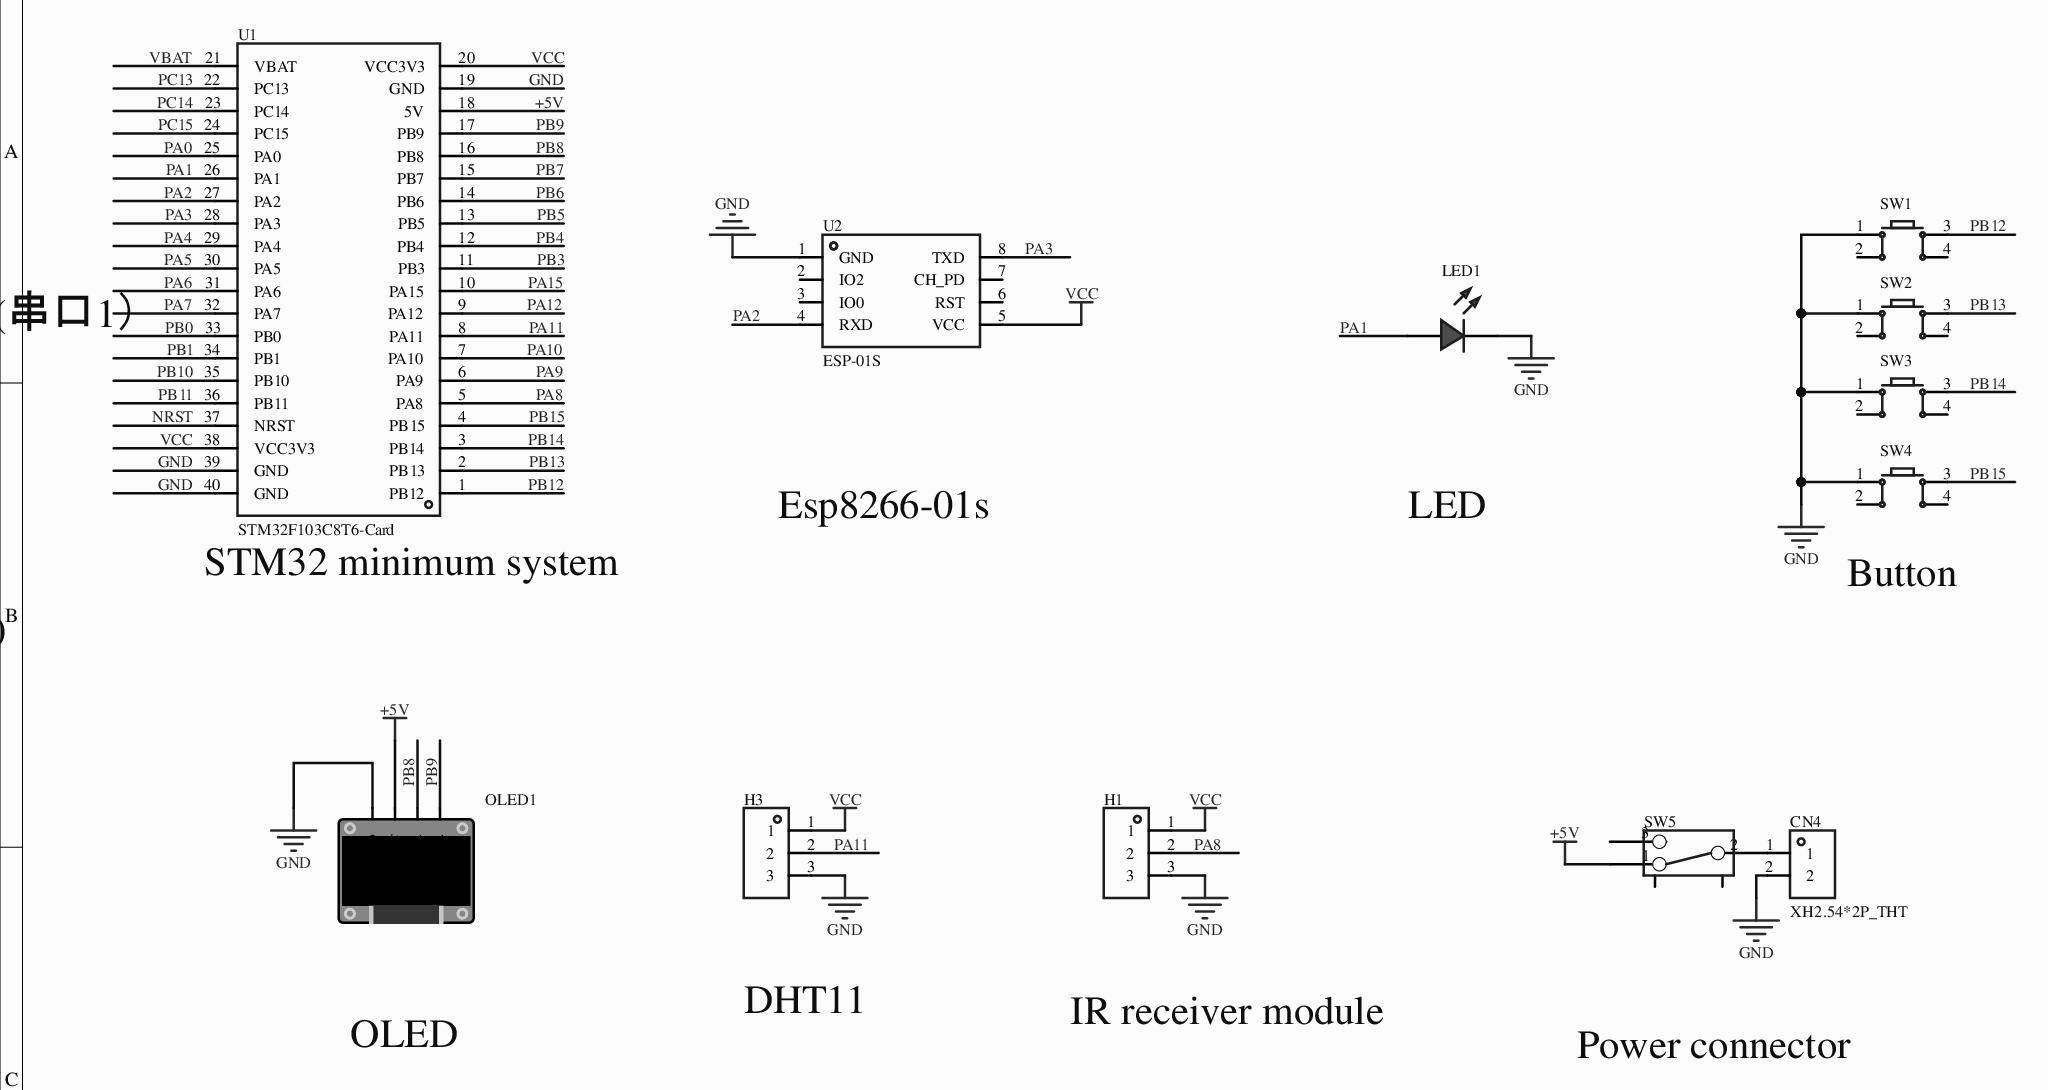
[diagram p0: MISC49868-3.schdoc]
# Altium project MISC49868-2.PrjPcb
1 sheet, 12 parts. Net scope: global (net labels, ports and power ports of the same name join across sheets).
Board file: MISC49868.pcbdoc

## Sheet MISC49868-3.schdoc
size 297 x 209 mm; Version: V1.0; @Project Name: MISC49868; @Page Count: 1; @Update Date: 2026-04-22; @Create Date: 2026-04-22; @Schematic Name: MISC49868; @Page No: 1; @Create Time: 23:22:16; @Update Time: 17:32:40; @Board Name: MISC49868

### Parts
CN4  XH2.54*2P_THT  [CONN-TH_2P-P2.50-XH2.54-2P]
H1  (no value)  [HDR-TH_3P-P2.54-V-F]
H3  (no value)  [HDR-TH_3P-P2.54-V-F]
LED1  (no value)  [LED-TH_5mm]
OLED1  (no value)  [0.96OLED_4P]
SW1  (no value)  [SW-TH_4P-L6.0-W6.0-P4.50-LS6.5]
SW2  (no value)  [SW-TH_4P-L6.0-W6.0-P4.50-LS6.5]
SW3  (no value)  [SW-TH_4P-L6.0-W6.0-P4.50-LS6.5]
SW4  (no value)  [SW-TH_4P-L6.0-W6.0-P4.50-LS6.5]
SW5  (no value)  [拨动开关]
U1  STM32F103C8T6-Card  [CONN-TH_L53.3-W22.9_STM32F103C8T6-CARD]
U2  ESP-01S  [WIFIM-TH_ESP-01S]

### Nets
+5V: OLED1.2(VCC) SW5.1 U1.18(5V)
GND: CN4.2 H1.3 H3.3 LED1.2(A) OLED1.1(GND) SW1.1 SW2.1 SW3.1 SW4.1 U1.19(GND) U1.39(GND) U1.40(GND) U2.1(GND)
VCC: H1.1 H3.1 U1.20(VCC3V3) U1.38(VCC3V3) U2.5(VCC)
NRST: U1.37(NRST)
PA0: U1.25(PA0)
PA1: LED1.1(C) U1.26(PA1)
PA2: U1.27(PA2) U2.4(RXD)
PA3: U1.28(PA3) U2.8(TXD)
PA4: U1.29(PA4)
PA5: U1.30(PA5)
PA6: U1.31(PA6)
PA7: U1.32(PA7)
PA8: H1.2 U1.5(PA8)
PA9: U1.6(PA9)
PA10: U1.7(PA10)
PA11: H3.2 U1.8(PA11)
PA12: U1.9(PA12)
PA15: U1.10(PA15)
PB0: U1.33(PB0)
PB1: U1.34(PB1)
PB3: U1.11(PB3)
PB4: U1.12(PB4)
PB5: U1.13(PB5)
PB6: U1.14(PB6)
PB7: U1.15(PB7)
PB8: OLED1.3(SCL) U1.16(PB8)
PB9: OLED1.4(SDA) U1.17(PB9)
PB10: U1.35(PB10)
PB11: U1.36(PB11)
PB12: SW1.3 U1.1(PB12)
PB13: SW2.3 U1.2(PB13)
PB14: SW3.3 U1.3(PB14)
PB15: SW4.3 U1.4(PB15)
PC13: U1.22(PC13)
PC14: U1.23(PC14)
PC15: U1.24(PC15)
VBAT: U1.21(VBAT)
NetCN4_1: CN4.1 SW5.2

Not connected (* = marked no-connect by the designer): SW1 2 4; SW2 2 4; SW3 2 4; SW4 2 4; SW5 3 4 5; U2 2(IO2)* 3(IO0)* 6(RST)* 7(CH_PD)*

### Notes on the sheet
- 串口：
  ESP8266-01s  		PA10，PA9 	(串口1）
  GPIO:
  LED灯	PA1
  按键：	PB1，P B2，P B3，P B4
  IIC:
  0.96英寸OLED显示屏	PB8(SCL)，PB9(SDA)
  One-Wire:
  DHT11 PA11
  NEC 协议：
  PB14
- (near U1) STM32 minimum system
- Esp8266-01s
- LED
- (near SW4) Button
- DHT11
- IR receiver module
- OLED
- Power connector

### Library data of the parts
CN4 = XH2.54*2P_直插: 3D Model: 325c595e30db4df8abe76612dd40b0fa0819f05c4eef4c71ace90d822a990e87; 3D Model Transform: 295.275,228.346,0,180,0,0,-0.002,-20.079,-137.795; AddInBom: yes; Device: XH2.54*2P_THT; Symbol: XH2.54*2P_THT; LCSC Part Name: XH2.54*2P_直插; Supplier Part: C9900008615; Manufacturer Part: XH2.54*2P_直插; Supplier Footprint: XH2.54_2P; JLCPCB Part Class: Extended Part; Supplier: LCSC; FootprintName: CONN-TH_2P-P2.50-XH2.54-2P; ConvertToPcb: yes; ModelName: CONN-TH_2P-P2.50-XH2.54-2P
H1 H3 = HDR-F_2.54_1x3P: Symbol: PM254V-11-03-H85; 3D Model: f3b3cc5aae9641bf9e56fc160cef875b; 3D Model Transform: 299.9994,100,0,0,0,0,0,0,-118.11; ConvertToPcb: yes; ModelName: HDR2.54-F-LI-1X3P; Device: HDR-F_2.54_1x3P; Supplier Part: C541850; Supplier Footprint: 插件; FootprintName: HDR-TH_3P-P2.54-V-F; AddInBom: yes
LED1 = LED_TH-R_5mm: ConvertToPcb: yes; ModelId: fe9cea1bdf7642cd8d9a5077ed0e2b580819f05c4eef4c71ace90d822a990e87; ModelName: LED-TH_BD5.9-P2.54-RD_RED; ModelTransform: 222.16,238.98,581.81,180,0,0,-6,0,-220; Symbol: LED_TH-R; Device: LED_TH-R_5mm; AddInBom: yes; FootprintName: LED-TH_5mm; Supplier Footprint: 插件
OLED1 = 0.96OLED模块_4P: Symbol: 0.96OLED module_4P; 3D Model: 79c000fdb68d45a296c2e9bedf4f9055; 3D Model Transform: 1393.69792,1318.895,0,0,0,0,0,-560.079,-137.795; ConvertToPcb: yes; Device: 0.96OLED module_4P; Supplier Footprint: 插件; AddInBom: yes; FootprintName: 0.96OLED_4P; ModelName: 0.96OLED_4P
SW1-SW4 = Key_TH_6x6x6: Contact current:50mA;Rated voltage(DC):12V;Insulation resistance:100MΩ;Circuit:SPST;Mounting:through-hole;Button shape:round;Button/cap colour:black;Actuation force:260gf@±30gf;Operating temperature:-25℃~+70℃;Pin style:PC pin;Switch length:6mm;Switch width:6mm;Switch height:6mm;With bracket:no;; Symbol: Tactile switch; AddInBom: yes; ModelId: 20eee248bc684ccd8cbdbb1d0d91ec6f0819f05c4eef4c71ace90d822a990e87; ModelName: SW-TH_4P-L6.0-W6.0-H5.0-LS6.5-P4.50; ModelTransform: 236.22,323.03,0,90,0,0,0,0,-137.795; Device: Key_TH_6x6x6; FootprintName: SW-TH_4P-L6.0-W6.0-P4.50-LS6.5; ConvertToPcb: yes; Supplier Footprint: 插件
SW5 = 拨动开关_正: Device: Toggle switch_pos; Symbol: Toggle switch; ConvertToPcb: yes; ModelId: 4321fe59a4074cbfb4989553f297c68f0819f05c4eef4c71ace90d822a990e87; ModelName: SW-TH_SS-12D02-VG4; ModelTransform: 370.09,208.7,472.35,0,0,0,0,0,-110; FootprintName: Toggle switch; AddInBom: yes; Supplier Footprint: 插件
U1 = STM32F103C8T6-Card: AddInBom: yes; Device: STM32F103C8T6-Card; Symbol: STM32F103C8T6-CARD; FootprintName: CONN-TH_L53.3-W22.9_STM32F103C8T6-CARD; LCSC Part Name: STM32F103C8T6-Card; SupplierPart: C9900077949; ManufacturerPart: STM32F103C8T6-Card; Supplier Footprint: 插件; Supplier: LCSC; ConvertToPcb: yes
U2 = ESP-01S_C111009: 3D Model: eb7175da78ae48b3b1568cfe3027405f0819f05c4eef4c71ace90d822a990e87; 3D Model Transform: 582.676,976.37608,0,0,0,0,0,388.346,-118.11; AddInBom: yes; Symbol: ESP-01S; Device: ESP-01S_C111009; LCSC Part Name: ESP-01S; Supplier Part: C111009; Manufacturer Part: ESP-01S; Supplier Footprint: -; JLCPCB Part Class: Extended Part; Supplier: LCSC; ConvertToPcb: yes; FootprintName: WIFIM-TH_ESP-01S; ModelName: WIFIM-TH_ESP-01S